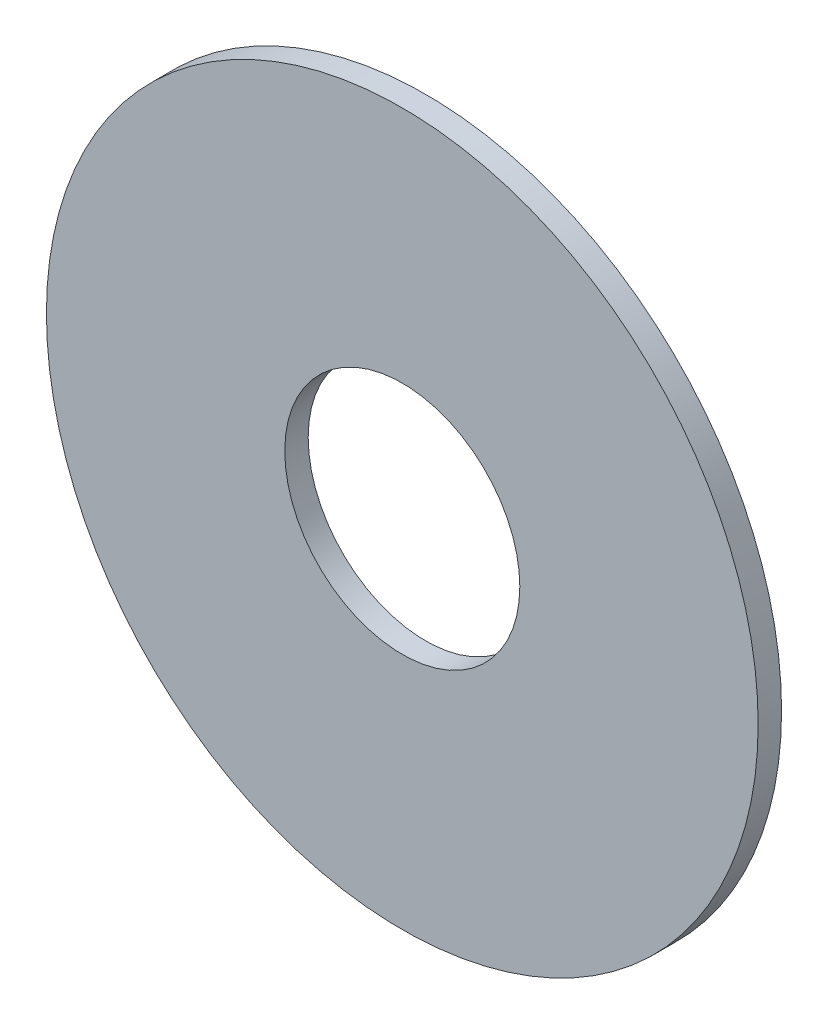
from build123d import *

# Parameters (mm, degrees)
SKETCH1_R           = 190
SKETCH1_R_2         = 62.75
BOSS_EXTRUDE1_DEPTH = 12.5


with BuildPart() as part:
    # Sketch1 → Boss-Extrude1 (new body)
    with BuildSketch(Plane.XY):
        Circle(SKETCH1_R)
        Circle(SKETCH1_R_2, mode=Mode.SUBTRACT)
    extrude(amount=BOSS_EXTRUDE1_DEPTH)


solid = part.part
